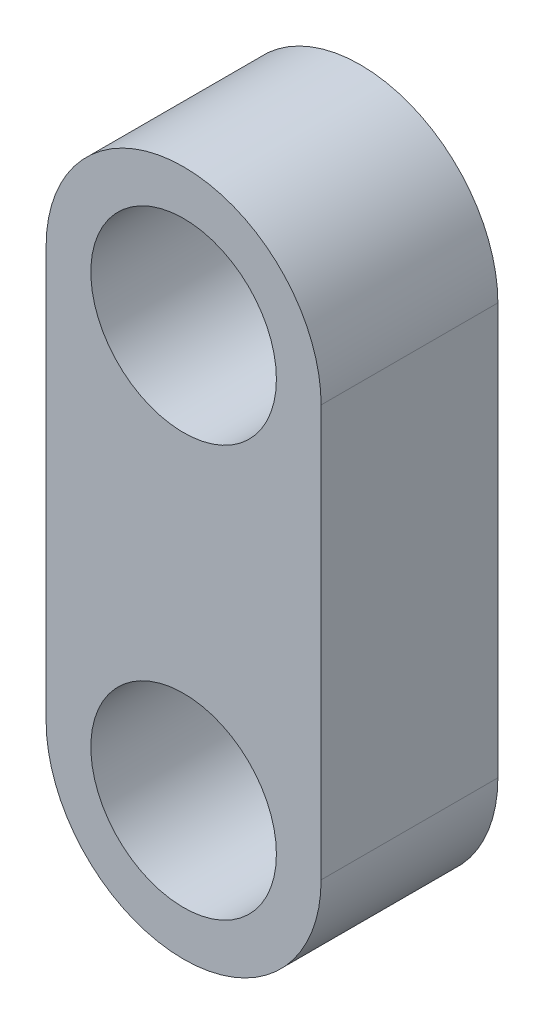
SolidWorks part; units mm, degrees
ref_plane "Front Plane" through (0, 0, 0) normal (0, 0, 1) x (1, 0, 0)
ref_plane "Top Plane" through (0, 0, 0) normal (0, 1, 0) x (1, 0, 0)
ref_plane "Right Plane" through (0, 0, 0) normal (1, 0, 0) x (0, 0, -1)
other "Configuration Table"
sketch "Sketch1" plane through (0, 0, 0) normal (0, 0, 1) x (1, 0, 0)
  line L0 (-32.5106, 16.2887) -> (-32.5106, 0)
  line L1 (-21.6207, 16.2887) -> (-21.6207, 0)
  arc A2 (-21.6207, 16.2887) -> (-32.5106, 16.2887) centre (-27.0657, 16.2887) ccw
  arc A3 (-32.5106, 0) -> (-21.6207, 0) centre (-27.0657, 0) ccw
extrude "Boss-Extrude2" add sketch "Sketch1" along normal mid plane 7 contours L0 A3 L1 A2
sketch "Sketch2" plane through (0, 0, 3.5) normal (0, 0, 1) x (1, 0, 0)
  circle A1 centre (-27.0657, 16.2887) radius 3.6746
sketch "Sketch4" plane through (0, 0, 3.5) normal (0, 0, 1) x (1, 0, 0)
  circle A0 centre (-27.0657, 0) radius 3.6746
extrude "Cut-Extrude1" cut sketch "Sketch4" against normal blind 10
extrude "Cut-Extrude2" cut sketch "Sketch2" against normal blind 10
